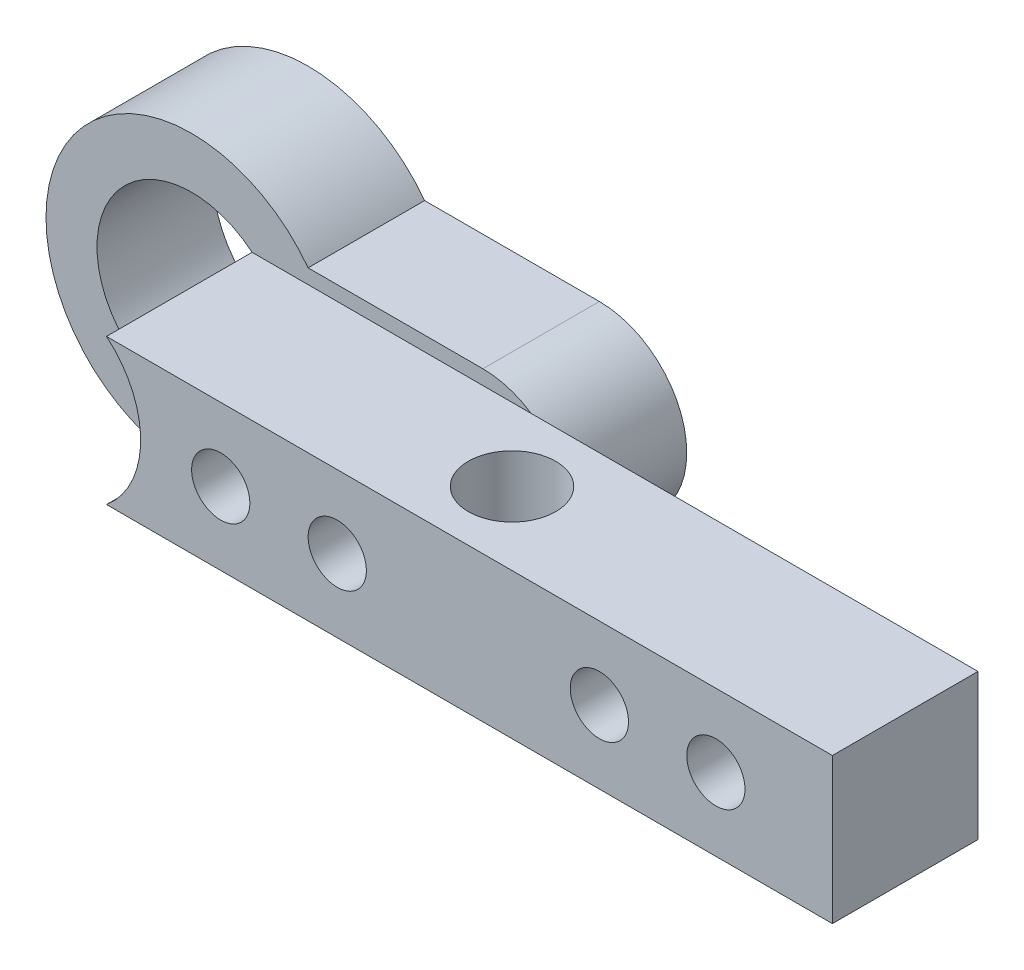
from build123d import *

# Parameters (mm, degrees)
SKETCH1_W               = 50
SKETCH1_H               = 10
BOSS_EXTRUDE1_DEPTH     = 10
SKETCH2_R               = 3
CUT_EXTRUDE1_DEPTH      = 10
SKETCH3_R               = 2
CUT_EXTRUDE2_DEPTH      = 10
BOSS_EXTRUDE2_DEPTH     = 30
CUT_EXTRUDE4_DEPTH      = 61.464865831
CUT_EXTRUDE4_DEPTH_BACK = 61.464865831
SKETCH6_W               = 47
SKETCH6_H               = 25
CUT_EXTRUDE5_DEPTH      = 54.150729064
CUT_EXTRUDE5_DEPTH_BACK = 54.150729064
SKETCH7_R               = 2
SKETCH5_R               = 6.5
CUT_EXTRUDE6_DEPTH      = 66.76473219


with BuildPart() as part:
    # Sketch1 → Boss-Extrude1 (new body)
    with BuildSketch(Plane(origin=(0, 0, 0), x_dir=(1, 0, 0), z_dir=(0, 1, 0))):
        with Locations((25, -5)):
            Rectangle(SKETCH1_W, SKETCH1_H)
    extrude(amount=BOSS_EXTRUDE1_DEPTH)

    # Sketch2 → Cut-Extrude1 (cut)
    with BuildSketch(Plane(origin=(0, 10, 0), x_dir=(1, 0, 0), z_dir=(0, 1, 0))):
        with Locations(Location((23, -5, 0), (0, 0, 270))):
            Circle(SKETCH2_R)
    extrude(amount=-CUT_EXTRUDE1_DEPTH, mode=Mode.SUBTRACT)

    # Sketch3 → Cut-Extrude2 (cut)
    with BuildSketch(Plane.XY.offset(10)):
        with Locations((8, 5)):
            Circle(SKETCH3_R)
        with Locations((16, 5)):
            Circle(SKETCH3_R)
        with Locations(Location((42, 5, 0), (0, 0, 180))):
            Circle(SKETCH3_R)
        with Locations(Location((34, 5, 0), (0, 0, 180))):
            Circle(SKETCH3_R)
    extrude(amount=-CUT_EXTRUDE2_DEPTH, mode=Mode.SUBTRACT)

    # Sketch4 → Boss-Extrude2 (add)
    with BuildSketch(Plane(origin=(0, 0, 0), x_dir=(-1, 0, 0), z_dir=(0, 0, -1))):
        with BuildLine():
            Line((-16, 11), (-4, 11))
            ThreePointArc((-4, 11), (14, 5), (-4, -1))
            Line((-4, -1), (-16, -1))
            ThreePointArc((-16, -1), (-22, 5), (-16, 11))
        make_face()
    extrude(amount=BOSS_EXTRUDE2_DEPTH)

    # Sketch6 → Cut-Extrude4 (cut, two sides: drawn at the far end of the back side and taken through both)
    with BuildSketch(Plane.XZ.offset(1).offset(-CUT_EXTRUDE4_DEPTH_BACK)):
        with Locations((4.191332745, -20.5)):
            Rectangle(SKETCH6_W, SKETCH6_H)
    extrude(amount=CUT_EXTRUDE4_DEPTH + CUT_EXTRUDE4_DEPTH_BACK, mode=Mode.SUBTRACT)

    # Sketch7 → Cut-Extrude5 (cut, two sides: drawn at the far end of the back side and taken through both)
    with BuildSketch(Plane.XY.offset(-CUT_EXTRUDE5_DEPTH_BACK)):
        with Locations((8, 5)):
            Circle(SKETCH7_R)
        with Locations((16, 5)):
            Circle(SKETCH7_R)
    extrude(amount=CUT_EXTRUDE5_DEPTH + CUT_EXTRUDE5_DEPTH_BACK, mode=Mode.SUBTRACT)

    # Sketch5 → Cut-Extrude6 (cut, through all)
    with BuildSketch(Plane(origin=(0, 0, -30), x_dir=(-1, 0, 0), z_dir=(0, 0, -1))):
        with Locations(Location((4, 5, 0), (0, 0, 230.284862768))):
            Circle(SKETCH5_R)
    extrude(amount=-CUT_EXTRUDE6_DEPTH, mode=Mode.SUBTRACT)


solid = part.part
